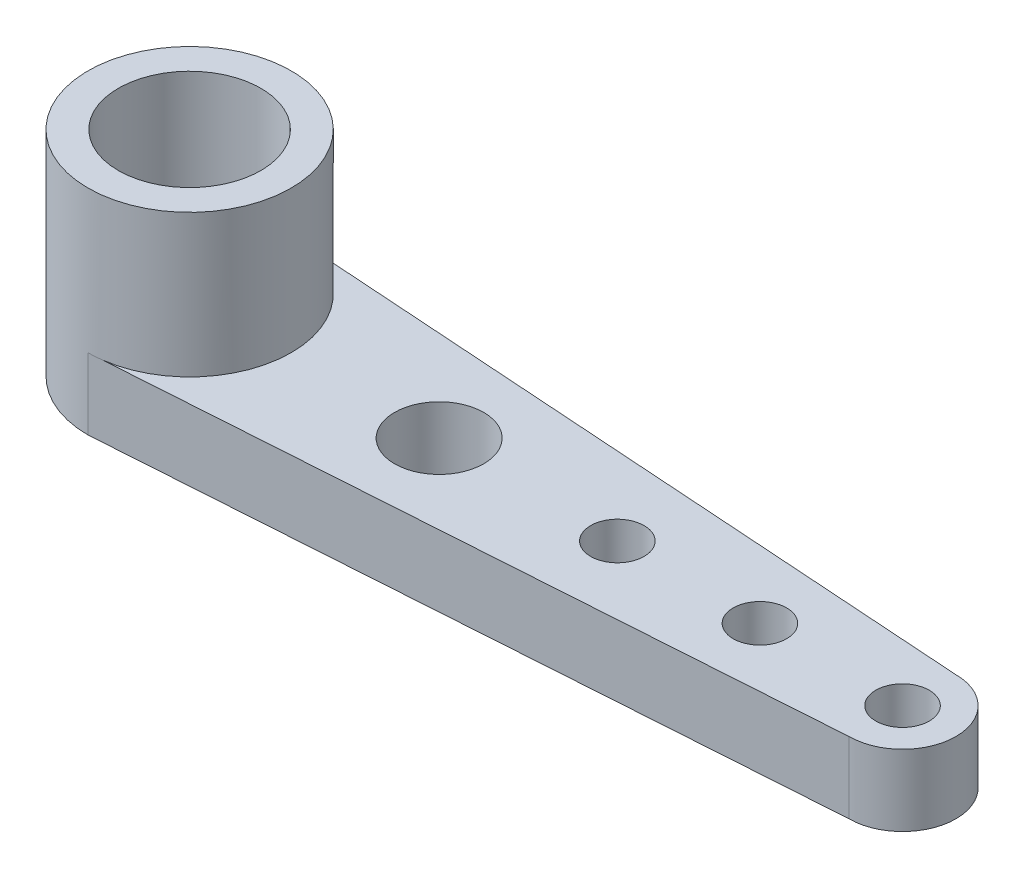
from build123d import *

# Parameters (mm, degrees)
BOSS_EXTRUDE1_DEPTH = 2
SKETCH2_R           = 2.85029491
SKETCH2_R_2         = 2
BOSS_EXTRUDE2_DEPTH = 4
SKETCH3_R           = 0.75
SKETCH3_R_2         = 1.25
CUT_EXTRUDE1_DEPTH  = 10


with BuildPart() as part:
    # Sketch1 → Boss-Extrude1 (new body)
    with BuildSketch(Plane(origin=(0, 0, 0), x_dir=(1, 0, 0), z_dir=(0, 1, 0))):
        with BuildLine():
            Line((0, 2.85029491), (20, 1.5))
            ThreePointArc((20, 1.5), (21.5, 0), (20, -1.5))
            Line((20, -1.5), (0, -2.85029491))
            ThreePointArc((0, -2.85029491), (-2.85029491, 0), (0, 2.85029491))
        make_face()
    extrude(amount=BOSS_EXTRUDE1_DEPTH)

    # Sketch2 → Boss-Extrude2 (add)
    with BuildSketch(Plane(origin=(0, 2, 0), x_dir=(1, 0, 0), z_dir=(0, 1, 0))):
        with Locations(Location((0, 0, 0), (0, 0, 270))):
            Circle(SKETCH2_R)
        with Locations(Location((0, 0, 0), (0, 0, 270))):
            Circle(SKETCH2_R_2, mode=Mode.SUBTRACT)
    extrude(amount=BOSS_EXTRUDE2_DEPTH)

    # Sketch3 → Cut-Extrude1 (cut)
    with BuildSketch(Plane.XZ):
        with Locations(Location((16, 0, 0), (0, 0, 270))):
            Circle(SKETCH3_R)
        with Locations(Location((12, 0, 0), (0, 0, 270))):
            Circle(SKETCH3_R)
        with Locations(Location((7, 0, 0), (0, 0, 270))):
            Circle(SKETCH3_R_2)
        with Locations(Location((20, 0, 0), (0, 0, 270))):
            Circle(SKETCH3_R)
    extrude(amount=-CUT_EXTRUDE1_DEPTH, mode=Mode.SUBTRACT)


solid = part.part
